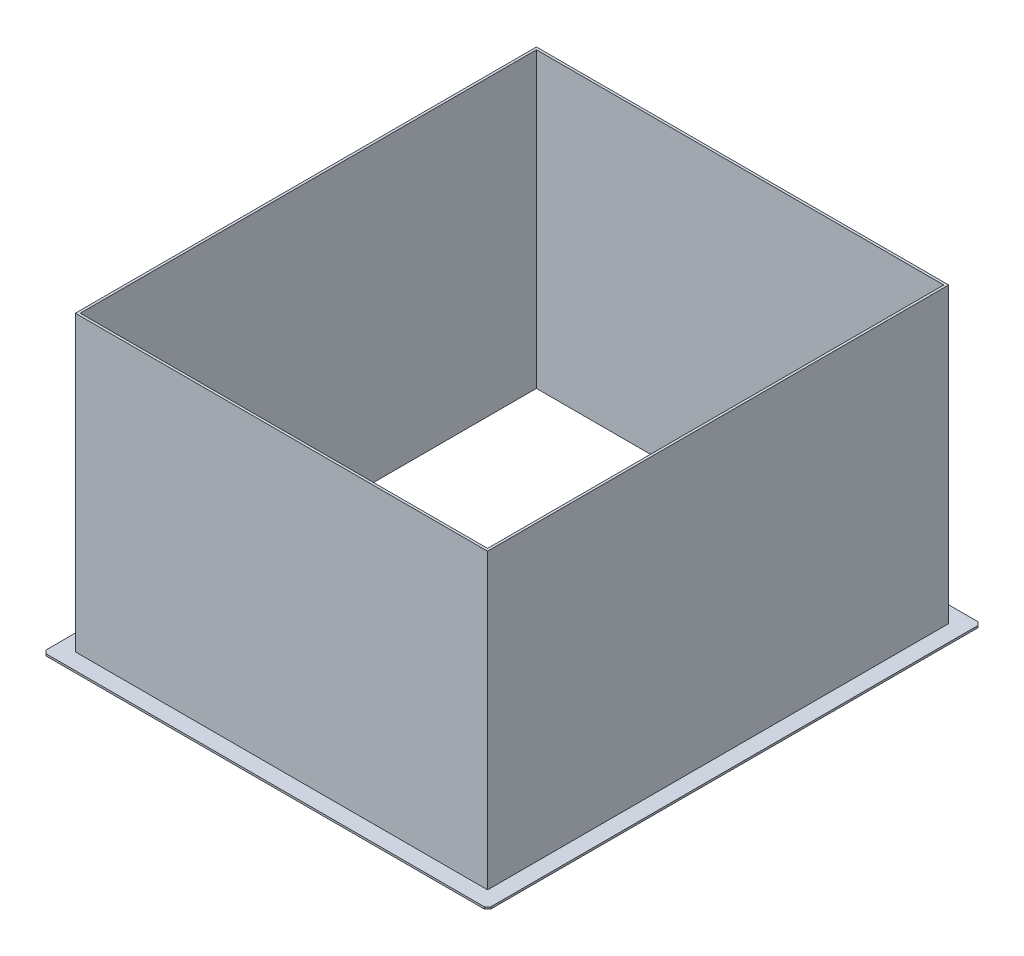
from build123d import *

# Parameters (mm, degrees)
SKETCH_1_W        = 253
SKETCH_1_H        = 283
SKETCH_1_W_2      = 250
SKETCH_1_H_2      = 280
EXTRUDE_1_DEPTH   = 180
SKETCH_2_W        = 273
SKETCH_2_H        = 303
SKETCH_2_W_2      = 253
SKETCH_2_H_2      = 283
EXTRUDE_1_2_DEPTH = 1.2
CHAMFER_1_SIZE    = 2


with BuildPart() as part:
    # 草图1 → Extrude 1 (new body)
    with BuildSketch(Plane(origin=(0, 0, 0), x_dir=(1, 0, 0), z_dir=(0, 1, 0))):
        Rectangle(SKETCH_1_W, SKETCH_1_H)
        Rectangle(SKETCH_1_W_2, SKETCH_1_H_2, mode=Mode.SUBTRACT)
    extrude(amount=EXTRUDE_1_DEPTH)


with BuildPart() as body_2:
    # 草图2 → Extrude 1 2 (new body)
    with BuildSketch(Plane.XZ):
        Rectangle(SKETCH_2_W, SKETCH_2_H)
        Rectangle(SKETCH_2_W_2, SKETCH_2_H_2, mode=Mode.SUBTRACT)
    extrude(amount=EXTRUDE_1_2_DEPTH)

    # 倒角1
    chamfer_1_edges = [body_2.edges().sort_by_distance(p)[0] for p in [
        (-136.5, -0.6, -151.5),
        (-136.5, -0.6, 151.5),
        (136.5, -0.6, 151.5),
        (136.5, -0.6, -151.5),
    ]]
    chamfer(chamfer_1_edges, length=CHAMFER_1_SIZE)


solid = Compound([part.part, body_2.part])
